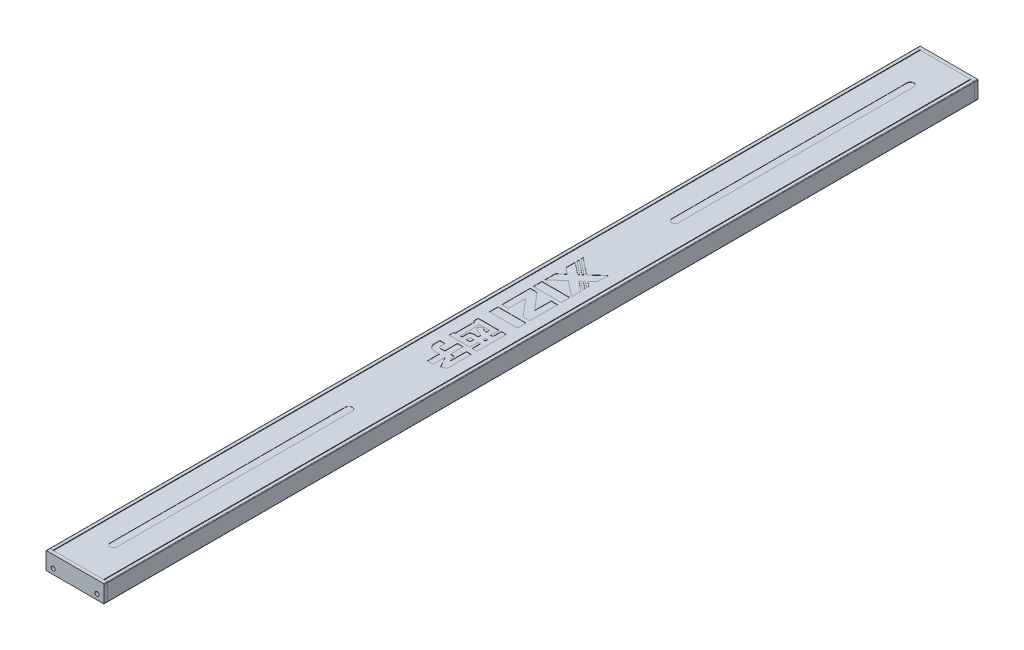
SolidWorks part; units mm, degrees
material "普通碳钢"
ref_plane "前视基准面" through (0, 0, 0) normal (0, 0, 1) x (1, 0, 0)
ref_plane "上视基准面" through (0, 0, 0) normal (0, 1, 0) x (1, 0, 0)
ref_plane "右视基准面" through (0, 0, 0) normal (1, 0, 0) x (0, 0, -1)
sketch "草图1" plane through (0, 0, 0) normal (0, 0, 1) x (1, 0, 0)
  line B0 (-21.0117, 7) -> (-23, 7)
  line B1 (-23, 7) -> (-23, 2)
  line B2 (-23, 2) -> (-21.0117, 2)
  line B3 (-21.0117, 2) -> (-21.0117, 2.8383)
  line B4 (-21.0117, 6.1617) -> (-21.0117, 7)
  line B5 (21.0117, 2.8383) -> (21.0117, 2)
  line B6 (21.0117, 2) -> (23, 2)
  line B7 (23, 2) -> (23, 7)
  line B8 (23, 7) -> (21.0117, 7)
  line B9 (21.0117, 7) -> (21.0117, 6.1617)
  line B10 (22, 15) -> (24.5, 15)
  line B11 (22, 15) -> (22, 9)
  line B12 (13, 9) -> (22, 9)
  line B13 (13, 9) -> (13, 8)
  line B14 (13, 8) -> (14.8, 8)
  line B15 (15, 7.8) -> (15, 2.7)
  line B16 (14.8, 2.5) -> (-14.8, 2.5)
  line B17 (-15, 7.8) -> (-15, 2.7)
  line B18 (-13, 8) -> (-14.8, 8)
  line B19 (-13, 9) -> (-13, 8)
  line B20 (-22, 9) -> (-13, 9)
  line B21 (-22, 9) -> (-22, 15)
  line B22 (-24.5, 15) -> (-22, 15)
  line B23 (-25, 0.5) -> (-25, 14.5)
  line B24 (-20.866, 0) -> (-24.5, 0)
  line B25 (-17.866, 0) -> (-19.134, 0)
  line B26 (-14.866, 0) -> (-16.134, 0)
  line B27 (-11.866, 0) -> (-13.134, 0)
  line B28 (10.134, 0) -> (-10.134, 0)
  line B29 (13.134, 0) -> (11.866, 0)
  line B30 (16.134, 0) -> (14.866, 0)
  line B31 (19.134, 0) -> (17.866, 0)
  line B32 (24.5, 0) -> (20.866, 0)
  line B33 (25, 14.5) -> (25, 0.5)
  arc B34 (-20.0728, 3.2272) -> (-21.0117, 2.8383) centre (-20.4617, 2.8383) ccw
  arc B35 (-20.0728, 3.2272) -> (-20.0728, 5.7728) centre (-18.8, 4.5) ccw
  arc B36 (-21.0117, 6.1617) -> (-20.0728, 5.7728) centre (-20.4617, 6.1617) ccw
  arc B37 (20.0728, 5.7728) -> (21.0117, 6.1617) centre (20.4617, 6.1617) ccw
  arc B38 (20.0728, 5.7728) -> (20.0728, 3.2272) centre (18.8, 4.5) ccw
  arc B39 (21.0117, 2.8383) -> (20.0728, 3.2272) centre (20.4617, 2.8383) ccw
  arc B40 (15, 7.8) -> (14.8, 8) centre (14.8, 7.8) ccw
  arc B41 (14.8, 2.5) -> (15, 2.7) centre (14.8, 2.7) ccw
  arc B42 (-15, 2.7) -> (-14.8, 2.5) centre (-14.8, 2.7) ccw
  arc B43 (-14.8, 8) -> (-15, 7.8) centre (-14.8, 7.8) ccw
  arc B44 (-24.5, 15) -> (-25, 14.5) centre (-24.5, 14.5) ccw
  arc B45 (-25, 0.5) -> (-24.5, 0) centre (-24.5, 0.5) ccw
  arc B46 (-19.134, 0) -> (-20.866, 0) centre (-20, -0.5) ccw
  arc B47 (-16.134, 0) -> (-17.866, 0) centre (-17, -0.5) ccw
  arc B48 (-13.134, 0) -> (-14.866, 0) centre (-14, -0.5) ccw
  arc B49 (-10.134, 0) -> (-11.866, 0) centre (-11, -0.5) ccw
  arc B50 (11.866, 0) -> (10.134, 0) centre (11, -0.5) ccw
  arc B51 (14.866, 0) -> (13.134, 0) centre (14, -0.5) ccw
  arc B52 (17.866, 0) -> (16.134, 0) centre (17, -0.5) ccw
  arc B53 (20.866, 0) -> (19.134, 0) centre (20, -0.5) ccw
  arc B54 (24.5, 0) -> (25, 0.5) centre (24.5, 0.5) ccw
  arc B55 (25, 14.5) -> (24.5, 15) centre (24.5, 14.5) ccw
sketch_block_instance "DFGDF SG343443-1"
sketch_block "DFGDF SG343443"
extrude "凸台-拉伸1" add sketch "草图1" along normal mid plane 744
sketch "草图3" plane through (0, 9, 363) normal (0, -1, 0) x (1, 0, 0)
  line L0 (-10.134, 9) -> (10.134, 9) construction
  line L5 (-21.5, -735) -> (21.5, -735)
  line L6 (-21.5, -735) -> (-21.5, 9)
  line L10 (-21.5, 9) -> (21.5, 9)
  line L11 (21.5, -735) -> (21.5, 9)
  line L12 (-21.5, -735) -> (21.5, 9) construction
  line L13 (-21.5, 9) -> (21.5, -735) construction
  line L14 (22, 9) -> (22, -735) construction
  point P0 (0, -363)
  dimension "D1" = 0.5
extrude "凸台-拉伸4" add sketch "草图3" against normal blind 6
sketch "草图7" plane through (0, 0, 372) normal (0, 0, 1) x (1, 0, 0)
  line L6 (-25, 14.5) -> (-25, 0.5) construction
  line L7 (-25, 15) -> (25, 15)
  line L8 (-25, 15) -> (-25, 0)
  line L9 (-25, 0) -> (25, 0)
  line L10 (25, 15) -> (25, 0)
  line L11 (-25, 15) -> (25, 0) construction
  line L12 (-25, 0) -> (25, 15) construction
  line L13 (25, 0.5) -> (25, 14.5) construction
  line L14 (-22, 15) -> (-24.5, 15) construction
  line L15 (-24.5, 0) -> (-20.866, 0) construction
  circle A2 centre (-18.8, 4.5) radius 1.75
  circle A3 centre (18.8, 4.5) radius 1.75
  point P0 (0, 7.5)
  dimension "D1" = 3.5
extrude "凸台-拉伸3" add sketch "草图7" along normal blind 3 separate body
mirror "镜向1" about plane through (0, 0, 0) normal (0, 0, 1) of bodies 111
fillet "圆角2" radius 0.5 4 edges at (-25, 0, 373.5) (-25, 15, 373.5) (25, 0, 373.5) (25, 15, 373.5)
fillet "圆角3" radius 0.5 4 edges at (-25, 0, -373.5) (-25, 15, -373.5) (25, 0, -373.5) (25, 15, -373.5)
sketch "草图13" plane through (0, 15, 0) normal (0, 1, 0) x (1, 0, 0)
  line L0 (0, 0) -> (-59.0386, 0) construction
  line L1 (2.9742, -342) -> (2.9742, -140)
  line L2 (-2.9742, -140) -> (-2.9742, -342)
  line L3 (0, 0) -> (0, 167.6847) construction
  line L127 (-2.9742, 140) -> (-2.9742, 342)
  line L128 (2.9742, 342) -> (2.9742, 140)
  line L184 (24.5, 372) -> (-24.5, 372) construction
  arc A0 (-2.9742, 140) -> (2.9742, 140) centre (0, 140) ccw
  arc A1 (2.9742, 342) -> (-2.9742, 342) centre (0, 342) ccw
  arc A2 (2.9742, -342) -> (-2.9742, -342) centre (0, -342) cw
  arc A3 (-2.9742, -140) -> (2.9742, -140) centre (0, -140) cw
  line B0 (4.4563, 54.7206) -> (12, 48.6925)
  line B1 (12, 48.6925) -> (12, 50.5773)
  line B2 (12, 50.5773) -> (5.5761, 55.7088)
  line B3 (5.5761, 55.7088) -> (6.471, 56.5041)
  line B4 (6.471, 56.5041) -> (12, 52.0887)
  line B5 (12, 52.0887) -> (12, 53.9736)
  line B6 (12, 53.9736) -> (7.5924, 57.4939)
  line B7 (7.5924, 57.4939) -> (12, 61.3922)
  line B8 (12, 61.3922) -> (12, 70.5504)
  line B9 (12, 70.5504) -> (2.1562, 61.8409)
  line B10 (2.1562, 61.8409) -> (-12, 73.1595)
  line B11 (-12, 73.1595) -> (-12, 71.2713)
  line B12 (-12, 71.2713) -> (1.0353, 60.8482)
  line B13 (1.0353, 60.8482) -> (0.1388, 60.0563)
  line B14 (0.1388, 60.0563) -> (-12, 69.7594)
  line B15 (-12, 69.7594) -> (-12, 67.8702)
  line B16 (-12, 67.8702) -> (-0.978, 59.063)
  line B17 (-0.978, 59.063) -> (-1.932, 58.2235)
  line B18 (-1.932, 58.2235) -> (-12, 66.2683)
  line B19 (-12, 66.2683) -> (-12, 58.2433)
  line B20 (-12, 58.2433) -> (-6.6975, 54.0095)
  line B21 (-6.6975, 54.0095) -> (-12, 49.3174)
  line B22 (-12, 49.3174) -> (-12, 40.1583)
  line B23 (-12, 40.1583) -> (-1.2567, 49.6603)
  line B24 (-1.2567, 49.6603) -> (12, 39.0655)
  line B25 (12, 39.0655) -> (12, 47.089)
  line B26 (12, 47.089) -> (3.5043, 53.8777)
  line B27 (3.5043, 53.8777) -> (4.4563, 54.7206)
  line B28 (-7.0911, 27.5607) -> (-12, 27.5607)
  line B29 (-12, 27.5607) -> (-12, 3.2556)
  line B30 (-12, 3.2556) -> (-6.3542, 3.2556)
  line B31 (-6.3542, 3.2556) -> (-6.3542, 18.0658)
  line B32 (-6.3542, 18.0658) -> (5.6412, 3.9436)
  line B33 (5.6412, 3.9436) -> (5.7204, 3.8804)
  line B34 (5.7204, 3.8804) -> (5.7998, 3.8179)
  line B35 (5.7998, 3.8179) -> (5.8798, 3.7568)
  line B36 (5.8798, 3.7568) -> (5.9607, 3.6979)
  line B37 (5.9607, 3.6979) -> (6.0426, 3.642)
  line B38 (6.0426, 3.642) -> (6.1259, 3.5897)
  line B39 (6.1259, 3.5897) -> (6.2109, 3.5418)
  line B40 (6.2109, 3.5418) -> (6.2978, 3.499)
  line B41 (6.2978, 3.499) -> (6.3869, 3.4621)
  line B42 (6.3869, 3.4621) -> (6.4785, 3.4316)
  line B43 (6.4785, 3.4316) -> (6.5723, 3.4071)
  line B44 (6.5723, 3.4071) -> (6.668, 3.3878)
  line B45 (6.668, 3.3878) -> (6.7654, 3.3728)
  line B46 (6.7654, 3.3728) -> (6.8641, 3.3612)
  line B47 (6.8641, 3.3612) -> (6.9638, 3.3522)
  line B48 (6.9638, 3.3522) -> (7.0641, 3.345)
  line B49 (7.0641, 3.345) -> (7.1647, 3.3385)
  line B50 (7.1647, 3.3385) -> (11.1965, 3.3385)
  line B51 (11.1965, 3.3385) -> (11.2237, 3.3399)
  line B52 (11.2237, 3.3399) -> (11.2508, 3.3414)
  line B53 (11.2508, 3.3414) -> (11.278, 3.343)
  line B54 (11.278, 3.343) -> (11.3051, 3.345)
  line B55 (11.3051, 3.345) -> (11.3321, 3.3472)
  line B56 (11.3321, 3.3472) -> (11.3591, 3.35)
  line B57 (11.3591, 3.35) -> (11.386, 3.3533)
  line B58 (11.386, 3.3533) -> (11.4127, 3.3573)
  line B59 (11.4127, 3.3573) -> (11.4394, 3.3619)
  line B60 (11.4394, 3.3619) -> (11.4659, 3.3674)
  line B61 (11.4659, 3.3674) -> (11.4922, 3.3739)
  line B62 (11.4922, 3.3739) -> (11.5184, 3.3811)
  line B63 (11.5184, 3.3811) -> (11.5443, 3.3893)
  line B64 (11.5443, 3.3893) -> (11.5699, 3.3984)
  line B65 (11.5699, 3.3984) -> (11.5952, 3.4084)
  line B66 (11.5952, 3.4084) -> (11.6202, 3.4193)
  line B67 (11.6202, 3.4193) -> (11.6447, 3.4311)
  line B68 (11.6447, 3.4311) -> (11.6688, 3.4437)
  line B69 (11.6688, 3.4437) -> (11.6925, 3.4573)
  line B70 (11.6925, 3.4573) -> (11.7155, 3.4717)
  line B71 (11.7155, 3.4717) -> (11.738, 3.4871)
  line B72 (11.738, 3.4871) -> (11.7598, 3.5033)
  line B73 (11.7598, 3.5033) -> (11.7808, 3.5204)
  line B74 (11.7808, 3.5204) -> (11.8011, 3.5383)
  line B75 (11.8011, 3.5383) -> (11.8206, 3.5572)
  line B76 (11.8206, 3.5572) -> (11.8392, 3.5769)
  line B77 (11.8392, 3.5769) -> (11.857, 3.5974)
  line B78 (11.857, 3.5974) -> (11.874, 3.6186)
  line B79 (11.874, 3.6186) -> (11.8901, 3.6406)
  line B80 (11.8901, 3.6406) -> (11.9053, 3.6632)
  line B81 (11.9053, 3.6632) -> (11.9197, 3.6864)
  line B82 (11.9197, 3.6864) -> (11.9331, 3.7102)
  line B83 (11.9331, 3.7102) -> (11.9455, 3.7346)
  line B84 (11.9455, 3.7346) -> (11.9567, 3.7595)
  line B85 (11.9567, 3.7595) -> (11.9668, 3.7848)
  line B86 (11.9668, 3.7848) -> (11.9755, 3.8105)
  line B87 (11.9755, 3.8105) -> (11.9827, 3.8366)
  line B88 (11.9827, 3.8366) -> (11.9886, 3.8631)
  line B89 (11.9886, 3.8631) -> (11.9931, 3.8898)
  line B90 (11.9931, 3.8898) -> (11.9968, 3.9167)
  line B91 (11.9968, 3.9167) -> (12, 3.9436)
  line B92 (12, 3.9436) -> (12, 27.158)
  line B93 (12, 27.158) -> (6.4203, 27.158)
  line B94 (6.4203, 27.158) -> (6.4203, 12.9362)
  line B95 (6.4203, 12.9362) -> (-5.1984, 26.5498)
  line B96 (-5.1984, 26.5498) -> (-5.2647, 26.619)
  line B97 (-5.2647, 26.619) -> (-5.3313, 26.688)
  line B98 (-5.3313, 26.688) -> (-5.3985, 26.7563)
  line B99 (-5.3985, 26.7563) -> (-5.4667, 26.8238)
  line B100 (-5.4667, 26.8238) -> (-5.536, 26.89)
  line B101 (-5.536, 26.89) -> (-5.6069, 26.9548)
  line B102 (-5.6069, 26.9548) -> (-5.6797, 27.0177)
  line B103 (-5.6797, 27.0177) -> (-5.7545, 27.0785)
  line B104 (-5.7545, 27.0785) -> (-5.8316, 27.1368)
  line B105 (-5.8316, 27.1368) -> (-5.9108, 27.1921)
  line B106 (-5.9108, 27.1921) -> (-5.9921, 27.2439)
  line B107 (-5.9921, 27.2439) -> (-6.0754, 27.2918)
  line B108 (-6.0754, 27.2918) -> (-6.1607, 27.3353)
  line B109 (-6.1607, 27.3353) -> (-6.248, 27.3739)
  line B110 (-6.248, 27.3739) -> (-6.337, 27.4075)
  line B111 (-6.337, 27.4075) -> (-6.4277, 27.4365)
  line B112 (-6.4277, 27.4365) -> (-6.5199, 27.4616)
  line B113 (-6.5199, 27.4616) -> (-6.6132, 27.4833)
  line B114 (-6.6132, 27.4833) -> (-6.7076, 27.5022)
  line B115 (-6.7076, 27.5022) -> (-6.8027, 27.5188)
  line B116 (-6.8027, 27.5188) -> (-6.8985, 27.5337)
  line B117 (-6.8985, 27.5337) -> (-6.9947, 27.5475)
  line B118 (-6.9947, 27.5475) -> (-7.0911, 27.5607)
  line B119 (12, 30.341) -> (12, 37.7143)
  line B120 (12, 37.7143) -> (-12, 37.7143)
  line B121 (-12, 37.7143) -> (-12, 30.341)
  line B122 (-12, 30.341) -> (12, 30.341)
  line B123 (-12, -7.3733) -> (12, -7.3733)
  line B124 (12, -7.3733) -> (12, 0)
  line B125 (12, 0) -> (-12, 0)
  line B126 (-12, 0) -> (-12, -7.3733)
  line B127 (5.9246, -28.7246) -> (5.9246, -30.5971)
  line B128 (5.9246, -30.5971) -> (7.818, -30.5971)
  line B129 (7.818, -30.5971) -> (7.818, -28.7246)
  line B130 (7.818, -28.7246) -> (5.9246, -28.7246)
  line B131 (-0.2616, -34.7893) -> (1.7387, -34.7893)
  line B132 (1.7387, -34.7893) -> (1.7387, -37.8582)
  line B133 (1.7387, -37.8582) -> (-1.3347, -37.8582)
  line B134 (-1.3347, -37.8582) -> (-1.3347, -35.8624)
  line B135 (5.9246, -24.169) -> (7.818, -24.169)
  line B136 (7.818, -24.169) -> (7.818, -16.9726)
  line B137 (7.818, -16.9726) -> (11.9826, -16.9726)
  line B138 (11.9826, -16.9726) -> (11.9826, -41.9704)
  line B139 (11.9826, -41.9704) -> (7.818, -41.9704)
  line B140 (7.818, -41.9704) -> (7.818, -34.7901)
  line B141 (7.818, -34.7901) -> (5.9246, -34.7901)
  line B142 (5.9246, -34.7901) -> (5.9246, -41.995)
  line B143 (5.9246, -41.995) -> (1.7387, -41.995)
  line B144 (1.7387, -41.995) -> (-12, -41.995)
  line B145 (-12, -41.995) -> (-12, -37.8582)
  line B146 (-12, -37.8582) -> (-10.85, -37.8582)
  line B147 (-10.85, -37.8582) -> (-10.85, -21.1325)
  line B148 (-10.85, -21.1325) -> (-12, -21.1325)
  line B149 (-12, -21.1325) -> (-12, -16.9733)
  line B150 (-12, -16.9733) -> (1.7387, -16.9733)
  line B151 (1.7387, -16.9733) -> (5.9246, -16.9733)
  line B152 (5.9246, -16.9733) -> (5.9246, -24.169)
  line B153 (1.7387, -23.831) -> (1.7387, -21.1325)
  line B154 (1.7387, -21.1325) -> (-6.6627, -21.1325)
  line B155 (-6.6627, -21.1325) -> (-6.6627, -37.8582)
  line B156 (-6.6627, -37.8582) -> (-5.1306, -37.8582)
  line B157 (-5.1306, -37.8582) -> (-5.1306, -33.3207)
  line B158 (-2.4479, -30.6379) -> (1.7387, -30.6379)
  line B159 (1.7387, -30.6379) -> (1.7387, -28.3543)
  line B160 (-5.7384, -24.1467) -> (-3.0617, -21.4527)
  line B161 (7.7102, -46.8925) -> (11.9598, -46.8925)
  line B162 (11.9598, -46.8925) -> (11.9598, -67.4971)
  line B163 (11.9598, -67.4971) -> (8.0857, -69.3711)
  line B164 (8.0857, -69.3711) -> (2.8273, -60.2214)
  line B165 (2.8273, -60.2214) -> (2.8273, -70.4521)
  line B166 (2.8273, -70.4521) -> (-2.1773, -70.4521)
  line B167 (-2.1773, -70.4521) -> (-2.1773, -60.1521)
  line B168 (-2.1773, -60.1521) -> (-6.5241, -60.1521)
  line B169 (-11.8897, -54.7866) -> (-11.8897, -49.9599)
  line B170 (-11.8897, -49.9599) -> (-7.3833, -49.9599)
  line B171 (-7.3833, -49.9599) -> (-7.3833, -54.2643)
  line B172 (-6.0419, -55.6057) -> (-2.1773, -55.6057)
  line B173 (-2.1773, -55.6057) -> (-2.1773, -44.6628)
  line B174 (-2.1773, -44.6628) -> (2.8273, -44.6628)
  line B175 (2.8273, -44.6628) -> (2.8273, -55.6057)
  line B176 (2.8273, -55.6057) -> (6.2535, -55.6057)
  line B177 (6.2535, -55.6057) -> (6.2535, -57.9509)
  line B178 (6.2535, -57.9509) -> (7.7102, -60.7865)
  line B179 (7.7102, -60.7865) -> (7.7102, -46.8925)
  arc B180 (-0.2616, -34.7893) -> (-1.3347, -35.8624) centre (-0.2616, -35.8624) ccw
  arc B181 (-3.0617, -21.4527) -> (1.7387, -23.831) centre (2.4693, -16.3225) ccw
  arc B182 (-2.4479, -30.6379) -> (-5.1306, -33.3207) centre (-2.4479, -33.3207) ccw
  arc B183 (-5.7384, -24.1467) -> (1.7387, -28.3543) centre (2.879, -17.5807) ccw
  arc B184 (-11.8897, -54.7866) -> (-6.5241, -60.1521) centre (-6.5241, -54.7866) ccw
  arc B185 (-7.3833, -54.2643) -> (-6.0419, -55.6057) centre (-6.0419, -54.2643) ccw
  dimension "D3" = 2.9742
  dimension "D1" = 30
  dimension "D2" = 140
sketch_block_instance "块2-1"
sketch_block "块2"
extrude "切除-拉伸1" cut sketch "草图13" against normal blind 0.2
